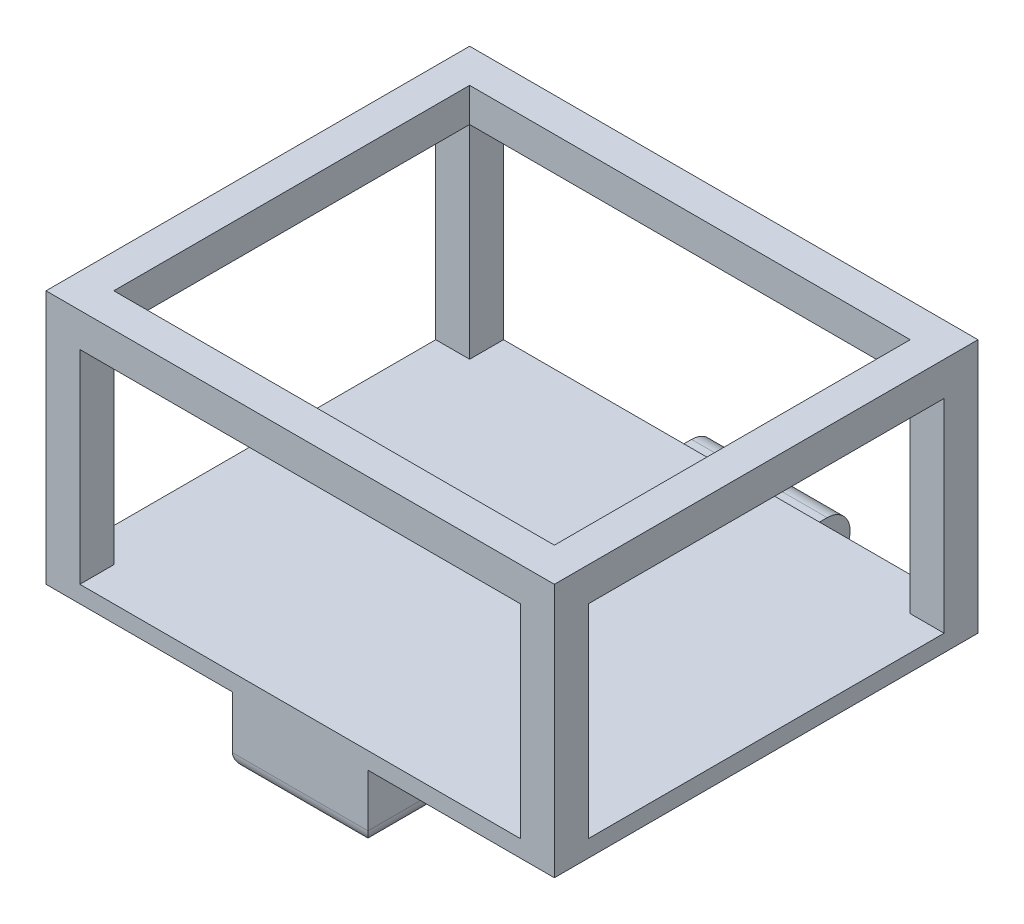
from build123d import *

# Parameters (mm, degrees)
SKETCH1_W           = 800
SKETCH1_H           = 400
BOSS_EXTRUDE1_DEPTH = 12500
SKETCH2_W           = 3000
SKETCH2_H           = 2500
BOSS_EXTRUDE2_DEPTH = 1500
SKETCH3_W           = 2100
SKETCH3_H           = 1200
CUT_EXTRUDE1_DEPTH  = 3000
SKETCH4_W           = 2600
SKETCH4_H           = 1200
CUT_EXTRUDE2_DEPTH  = 3000
SKETCH5_W           = 2600
SKETCH5_H           = 2100
CUT_EXTRUDE3_DEPTH  = 1000
FILLET1_R           = 90
SKETCH6_W           = 1631.27980794
SKETCH6_H           = 982.131348286
CUT_EXTRUDE4_DEPTH  = 10254.779790887
BOSS_EXTRUDE3_REACH = 12759.351


with BuildPart() as part:
    # Sketch1 → Boss-Extrude1 (new body)
    with BuildSketch(Plane.XY):
        Rectangle(SKETCH1_W, SKETCH1_H)
    extrude(amount=BOSS_EXTRUDE1_DEPTH)

    # Sketch2 → Boss-Extrude2 (add)
    with BuildSketch(Plane(origin=(0, 200, 0), x_dir=(1, 0, 0), z_dir=(0, 1, 0))):
        with Locations((0, -11250)):
            Rectangle(SKETCH2_W, SKETCH2_H)
    extrude(amount=BOSS_EXTRUDE2_DEPTH)

    # Sketch3 → Cut-Extrude1 (cut)
    with BuildSketch(Plane(origin=(1500, 0, 0), x_dir=(0, 0, -1), z_dir=(1, 0, 0))):
        with Locations((-11250, 900)):
            Rectangle(SKETCH3_W, SKETCH3_H)
    extrude(amount=-CUT_EXTRUDE1_DEPTH, mode=Mode.SUBTRACT)

    # Sketch4 → Cut-Extrude2 (cut)
    with BuildSketch(Plane(origin=(0, 0, 10000), x_dir=(-1, 0, 0), z_dir=(0, 0, -1))):
        with Locations((0, 900)):
            Rectangle(SKETCH4_W, SKETCH4_H)
    extrude(amount=-CUT_EXTRUDE2_DEPTH, mode=Mode.SUBTRACT)

    # Sketch5 → Cut-Extrude3 (cut)
    with BuildSketch(Plane(origin=(0, 1700, 0), x_dir=(1, 0, 0), z_dir=(0, 1, 0))):
        with Locations((0, -11250)):
            Rectangle(SKETCH5_W, SKETCH5_H)
    extrude(amount=-CUT_EXTRUDE3_DEPTH, mode=Mode.SUBTRACT)

    # Fillet1
    fillet1_edges = [part.edges().sort_by_distance(p)[0] for p in [
        (-400, 200, 5000),
        (400, 200, 5000),
        (0, -200, 12500),
        (400, -200, 6250),
        (-400, -200, 6250),
    ]]
    fillet(fillet1_edges, radius=FILLET1_R)

    # Sketch6 → Cut-Extrude4 (cut, through all)
    with BuildSketch(Plane(origin=(0, 0, 10000), x_dir=(-1, 0, 0), z_dir=(0, 0, -1))):
        with Locations((-94.176978603, 201.755445991)):
            Rectangle(SKETCH6_W, SKETCH6_H)
    extrude(amount=CUT_EXTRUDE4_DEPTH, mode=Mode.SUBTRACT)

    # Boss-Extrude3: up to this face of the body (flat: up to its plane)
    boss_extrude3_end = Plane(part.part.faces().sort_by_distance((-400, 45, 11250))[0])
    # Sketch7 → Boss-Extrude3 (add, up to the picked face)
    with BuildSketch(Plane(origin=(400, 0, 0), x_dir=(0, 0, -1), z_dir=(1, 0, 0)), mode=Mode.PRIVATE) as boss_extrude3_sk1:
        with BuildLine():
            Line((-10304.132937167, 135.712060669), (-9790.263777043, 135.712060669))
            ThreePointArc((-9790.263777043, 135.712060669), (-9654.551716374, 0), (-9790.263777043, -135.712060669))
            Line((-9790.263777043, -135.712060669), (-10304.132937167, -135.712060669))
            ThreePointArc((-10304.132937167, -135.712060669), (-10439.844997836, 0), (-10304.132937167, 135.712060669))
        make_face()
    boss_extrude3_tool1 = split(extrude(boss_extrude3_sk1.sketch, amount=-BOSS_EXTRUDE3_REACH, mode=Mode.PRIVATE), bisect_by=boss_extrude3_end, keep=Keep.BOTH, mode=Mode.PRIVATE)
    add(boss_extrude3_tool1.solids().sort_by(Axis((400, 0, 10047.198357), (-1, 0, 0)))[0])


solid = part.part
